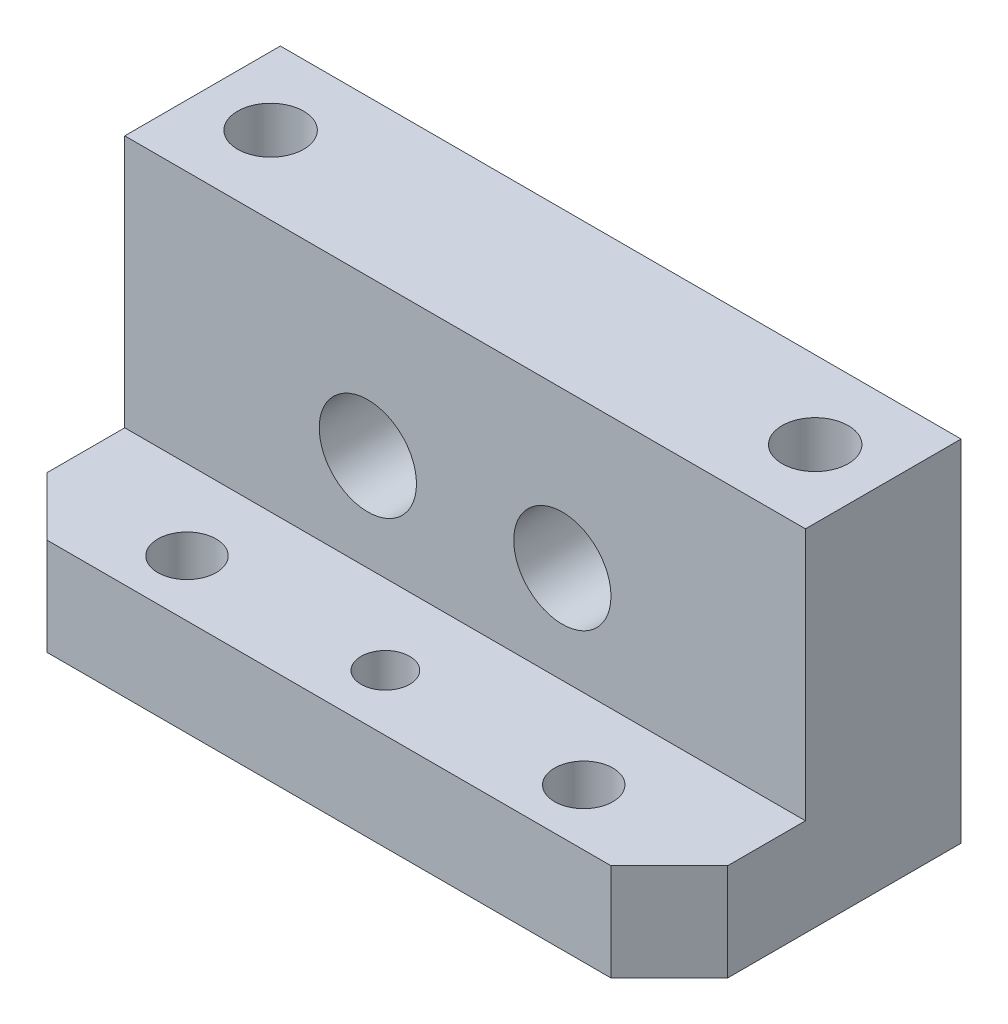
from build123d import *

# Parameters (mm, degrees)
SKETCH1_W                                            = 35
SKETCH1_H                                            = 18
BOSS_EXTRUDE1_DEPTH                                  = 7.5
SKETCH2_W                                            = 7
SKETCH2_H                                            = 13
CUT_EXTRUDE1_DEPTH                                   = 37.908671068
F_5_0_5_DIAMETER_HOLE1_D                             = 5
F_3_0_3_DIAMETER_HOLE2_D                             = 3
F_3_0_3_DIAMETER_HOLE2_DEPTH                         = 3
F_3_0_3_DIAMETER_HOLE2_TIP                           = 0.901290929
M3_TAPPED_HOLE1_D                                    = 2.5
HOLE_SIZE_PER_SOCKET_HEAD_CAP_SCREW_TYPE_D           = 3.4
HOLE_SIZE_PER_SOCKET_HEAD_CAP_SCREW_TYPE_CBORE_D     = 6
HOLE_SIZE_PER_SOCKET_HEAD_CAP_SCREW_TYPE_CBORE_DEPTH = 5
CHAMFER1_SIZE                                        = 3


with BuildPart() as part:
    # Sketch1 → Boss-Extrude1 (new, symmetric)
    with BuildSketch(Plane.XY):
        Rectangle(SKETCH1_W, SKETCH1_H)
    extrude(amount=BOSS_EXTRUDE1_DEPTH, both=True)

    # Sketch2 → Cut-Extrude1 (cut, through all)
    with BuildSketch(Plane(origin=(17.5, 0, 0), x_dir=(0, 0, -1), z_dir=(1, 0, 0))):
        with Locations((-4, 2.5)):
            Rectangle(SKETCH2_W, SKETCH2_H)
    extrude(amount=-CUT_EXTRUDE1_DEPTH, mode=Mode.SUBTRACT)

    # Ø5.0 (5) Diameter Hole1 (through all)
    with Locations(Plane.XY.offset(0.5)):
        with Locations((-5, 1), (5, 1)):
            Hole(F_5_0_5_DIAMETER_HOLE1_D / 2)

    # Ø3.0 (3) Diameter Hole2
    with Locations(Plane(origin=(0, -4, 0), x_dir=(1, 0, 0), z_dir=(0, 1, 0))):
        with Locations((10.2, -4.6), (-10.2, -4.6)):
            Hole(F_3_0_3_DIAMETER_HOLE2_D / 2, depth=F_3_0_3_DIAMETER_HOLE2_DEPTH)
            with Locations((0, 0, -(F_3_0_3_DIAMETER_HOLE2_DEPTH + F_3_0_3_DIAMETER_HOLE2_TIP / 2))):  # 118° drill point
                Cone(0, F_3_0_3_DIAMETER_HOLE2_D / 2, F_3_0_3_DIAMETER_HOLE2_TIP, mode=Mode.SUBTRACT)

    # M3 Tapped Hole1 (through all)
    with Locations(Plane(origin=(0, -9, 0), x_dir=(-1, 0, 0), z_dir=(0, -1, 0))):
        with Locations((0, -4.6)):
            Hole(M3_TAPPED_HOLE1_D / 2)

    # Hole size per socket head cap screw type1 (through all)
    with Locations(Plane(origin=(0, -9, 0), x_dir=(-1, 0, 0), z_dir=(0, -1, 0))):
        with Locations((14, 3.5), (-14, 3.5)):
            CounterBoreHole(HOLE_SIZE_PER_SOCKET_HEAD_CAP_SCREW_TYPE_D / 2, HOLE_SIZE_PER_SOCKET_HEAD_CAP_SCREW_TYPE_CBORE_D / 2, HOLE_SIZE_PER_SOCKET_HEAD_CAP_SCREW_TYPE_CBORE_DEPTH)

    # Chamfer1
    chamfer1_edges = [part.edges().sort_by_distance(p)[0] for p in [
        (-17.5, -6.5, 7.5),
        (17.5, -6.5, 7.5),
    ]]
    chamfer(chamfer1_edges, length=CHAMFER1_SIZE)


solid = part.part
